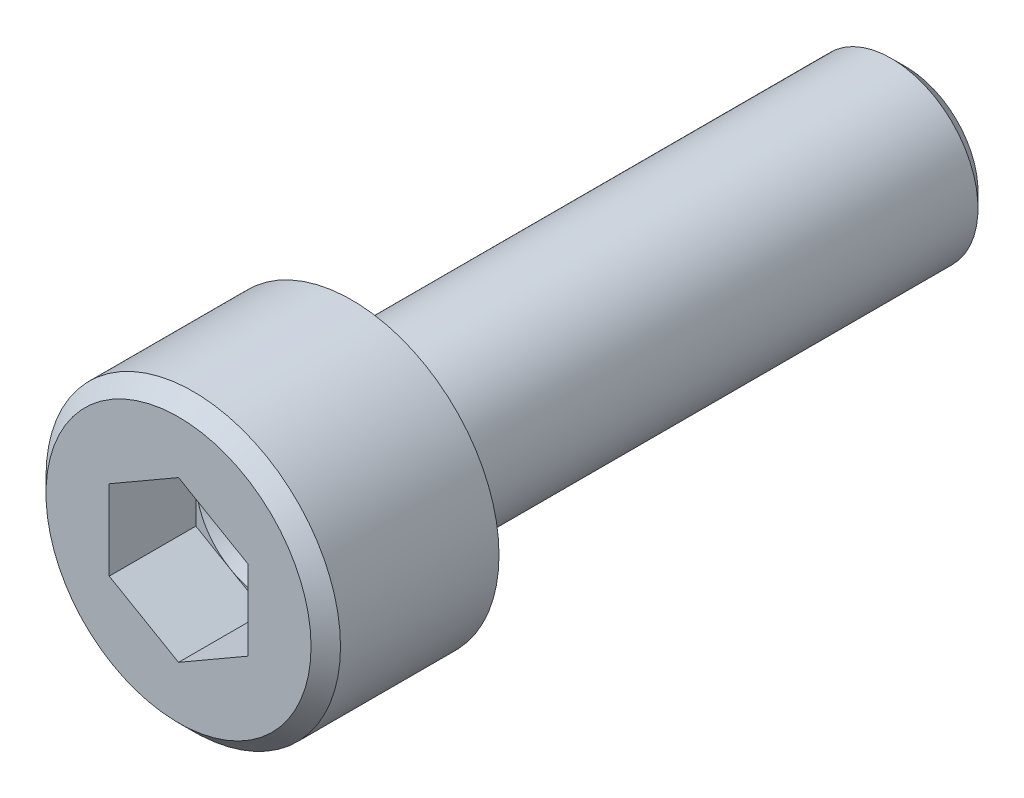
SolidWorks part; units mm, degrees
material "SUS304/0Cr18Ni9"
ref_plane "前视基准面" through (0, 0, 0) normal (0, 0, 1) x (1, 0, 0)
ref_plane "上视基准面" through (0, 0, 0) normal (0, 1, 0) x (1, 0, 0)
ref_plane "右视基准面" through (0, 0, 0) normal (1, 0, 0) x (0, 0, -1)
sketch "草图1" plane through (0, 0, 0) normal (0, 1, 0) x (1, 0, 0)
  line L0 (4.25, 0) -> (0, 0)
  line L1 (0, 0) -> (0, -5)
  line L2 (0, -5) -> (4.25, -5)
  line L3 (4.25, -5) -> (4.25, 0)
  line L4 (0, 0) -> (0, -5) construction
revolve "旋转1" add sketch "草图1" angle 360 about L4
sketch "草图2" plane through (0, 0, 0) normal (0, 0, -1) x (-1, 0, 0)
  circle A0 centre (0, 0) radius 2.5
extrude "凸台-拉伸1" add sketch "草图2" along normal blind 16
sketch "草图3" plane through (0, 0, 5) normal (0, 0, 1) x (1, 0, 0)
  line L0 (2, 1.1547) -> (0, 2.3094)
  line L1 (0, 2.3094) -> (-2, 1.1547)
  line L2 (-2, 1.1547) -> (-2, -1.1547)
  line L3 (-2, -1.1547) -> (0, -2.3094)
  line L4 (0, -2.3094) -> (2, -1.1547)
  line L5 (2, -1.1547) -> (2, 1.1547)
extrude "切除-拉伸1" cut sketch "草图3" against normal blind 2.5
ref_plane "基准面1" through (0, 0, 0) normal (0, -1, 0) x (1, 0, 0)
sketch "草图4" plane through (0, 0, 0) normal (0, -1, 0) x (1, 0, 0)
  line L0 (2, 2.5) -> (0, 2.5)
  line L1 (0, 2.5) -> (0, 1.3453)
  line L2 (0, 1.3453) -> (2, 2.5)
  line L3 (0, 2.5) -> (0, 1.3453) construction
revolve "切除-旋转1" cut sketch "草图4" angle 360 about L3
chamfer "倒角1" distance 0.425 angle 45 2 edges at (-2.5, 0, -16) (4.25, 0, 5)
